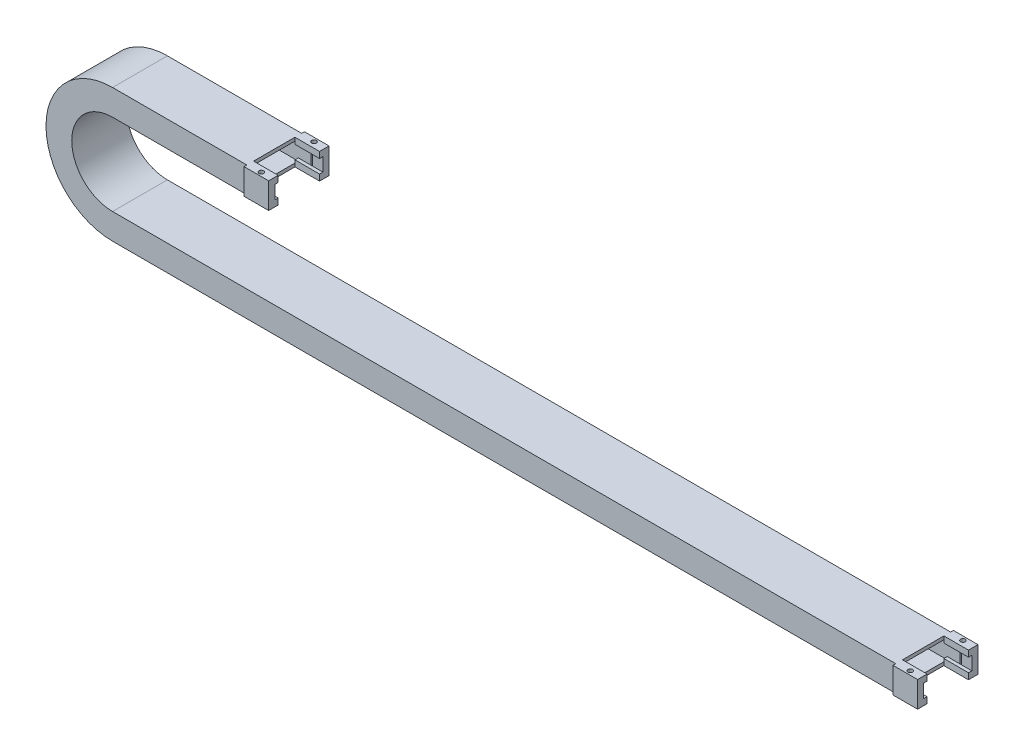
SolidWorks part; units mm, degrees
ref_plane "前视基准面" through (0, 0, 0) normal (0, 0, 1) x (1, 0, 0)
ref_plane "上视基准面" through (0, 0, 0) normal (0, 1, 0) x (1, 0, 0)
ref_plane "右视基准面" through (0, 0, 0) normal (1, 0, 0) x (0, 0, -1)
sketch "草图1" plane through (0, 0, 0) normal (0, 0, 1) x (1, 0, 0)
  line L0 (0, 0) -> (-700, 0)
  line L1 (-700, 96) -> (-580, 96)
  arc A0 (-700, 96) -> (-700, 0) centre (-700, 48) ccw
  dimension "D2" = 48
  dimension "D1" = 700
  dimension "D3" = 120
sketch "草图2" plane through (0, 0, 0) normal (1, 0, 0) x (0, 0, -1)
  line L1 (24.5, 11.5) -> (-24.5, 11.5)
  line L2 (24.5, 11.5) -> (24.5, -11.5)
  line L3 (24.5, -11.5) -> (-24.5, -11.5)
  line L4 (-24.5, 11.5) -> (-24.5, -11.5)
  line L5 (24.5, 11.5) -> (-24.5, -11.5) construction
  line L6 (24.5, -11.5) -> (-24.5, 11.5) construction
  point P0 (0, 0)
  dimension "D1" = 23
  dimension "D2" = 49
sweep "扫描1" add profiles "草图2" path "草图1"
shell "抽壳1" thickness 3
sketch "草图3" plane through (0, 11.5, 0) normal (0, 1, 0) x (1, 0, 0)
  line L0 (-7, 7.5) -> (-7, -7.5) construction
  line L1 (0, 0) -> (-7, 0) construction
  line L2 (0, 24.5) -> (0, -24.5) construction
  circle A0 centre (-7, 7.5) radius 2.5
  circle A1 centre (-7, -7.5) radius 2.5
  dimension "D2" = 7
  dimension "D1" = 5
  dimension "D3" = 15
extrude "切除-拉伸1" [suppressed] cut sketch "草图3" against normal through all
sketch "草图4" plane through (0, 107.5, 0) normal (0, 1, 0) x (1, 0, 0)
  line L0 (-587, 7.5) -> (-587, -7.5) construction
  line L1 (-587, 0) -> (-580, 0) construction
  line L2 (-580, -24.5) -> (-580, 24.5) construction
  circle A0 centre (-587, 7.5) radius 2.5
  circle A1 centre (-587, -7.5) radius 2.5
  dimension "D1" = 15
  dimension "D2" = 5
  dimension "D3" = 7
extrude "切除-拉伸2" [suppressed] cut sketch "草图4" against normal up to surface (24 mm away)
sketch "草图5" plane through (0, 11.5, 0) normal (0, 1, 0) x (1, 0, 0)
  line L0 (0, 24.5) -> (0, -24.5) construction
  line L1 (-40, 21) -> (25.9694, 21)
  line L2 (-40, 21) -> (-40, -21)
  line L3 (-40, -21) -> (25.9694, -21)
  line L4 (25.9694, 21) -> (25.9694, -21)
  line L5 (-40, 21) -> (25.9694, -21) construction
  line L6 (-40, -21) -> (25.9694, 21) construction
  point P0 (-7.0153, 0)
  dimension "D1" = 42
  dimension "D2" = 40
extrude "切除-拉伸3" [suppressed] cut sketch "草图5" against normal blind 5
sketch "草图6" plane through (0, 0, 24.5) normal (0, 0, 1) x (1, 0, 0)
  line L0 (-20, 11.5) -> (0, 1.5)
  line L1 (-700, 11.5) -> (0, 11.5) construction
  line L2 (0, 11.5) -> (0, -11.5) construction
  line L3 (0, 1.5) -> (0, 11.5)
  line L4 (0, 11.5) -> (-20, 11.5)
  dimension "D1" = 20
  dimension "D2" = 10
extrude "切除-拉伸4" [suppressed] cut sketch "草图6" against normal through all
fillet "圆角1" [suppressed] radius 5
sketch "草图7" plane through (0, -8.5, 0) normal (0, 1, 0) x (1, 0, 0)
  line L0 (0, -21.5) -> (0, 21.5) construction
  line L1 (-39, 18.5) -> (-25, 18.5)
  line L2 (-39, 18.5) -> (-39, -18.5)
  line L3 (-39, -18.5) -> (-25, -18.5)
  line L4 (-25, 18.5) -> (-25, -18.5)
  line L5 (-39, 18.5) -> (-25, -18.5) construction
  line L6 (-39, -18.5) -> (-25, 18.5) construction
  point P0 (-32, 0)
  dimension "D1" = 14
  dimension "D2" = 37
  dimension "D3" = 25
extrude "切除-拉伸5" [suppressed] cut sketch "草图7" against normal blind 5
sketch "草图8" plane through (0, 104.5, 0) normal (0, -1, 0) x (1, 0, 0)
  line L0 (-580, -24.5) -> (-580, 24.5) construction
  line L1 (-620, 21) -> (-279.3779, 21)
  line L2 (-620, 21) -> (-620, -21)
  line L3 (-620, -21) -> (-279.3779, -21)
  line L4 (-279.3779, 21) -> (-279.3779, -21)
  line L5 (-620, 21) -> (-279.3779, -21) construction
  line L6 (-620, -21) -> (-279.3779, 21) construction
  point P0 (-449.689, 0)
  dimension "D1" = 42
  dimension "D2" = 40
extrude "切除-拉伸6" [suppressed] cut sketch "草图8" against normal blind 5
sketch "草图9" plane through (0, 0, 24.5) normal (0, 0, 1) x (1, 0, 0)
  line L0 (-580, 97.5) -> (-580, 107.5)
  line L1 (-580, 84.5) -> (-580, 107.5) construction
  line L3 (-580, 107.5) -> (-600, 107.5)
  line L4 (-700, 107.5) -> (-580, 107.5) construction
  line L5 (-600, 107.5) -> (-580, 97.5)
  dimension "D1" = 10
  dimension "D2" = 20
extrude "切除-拉伸7" [suppressed] cut sketch "草图9" against normal through all
fillet "圆角2" [suppressed] radius 5
sketch "草图10" plane through (0, 87.5, 0) normal (0, 1, 0) x (1, 0, 0)
  line L0 (-580, -24.5) -> (-580, 24.5) construction
  line L1 (-605, -18.5) -> (-619, -18.5)
  line L2 (-605, -18.5) -> (-605, 18.5)
  line L3 (-605, 18.5) -> (-619, 18.5)
  line L4 (-619, -18.5) -> (-619, 18.5)
  line L5 (-605, -18.5) -> (-619, 18.5) construction
  line L6 (-605, 18.5) -> (-619, -18.5) construction
  point P0 (-612, 0)
  dimension "D1" = 37
  dimension "D2" = 14
  dimension "D3" = 25
extrude "切除-拉伸8" [suppressed] cut sketch "草图10" against normal blind 5
sketch "草图11" plane through (0, 0, 0) normal (1, 0, 0) x (0, 0, -1)
  line L0 (24.5, 11.5) -> (-24.5, 11.5) construction
  line L1 (-27, 11.5) -> (27, 11.5)
  line L2 (-27, 11.5) -> (-27, -11.5)
  line L3 (-27, -11.5) -> (27, -11.5)
  line L4 (27, 11.5) -> (27, -11.5)
  line L5 (-27, 11.5) -> (27, -11.5) construction
  line L6 (-27, -11.5) -> (27, 11.5) construction
  line L7 (-21.5, 6) -> (21.5, 6)
  line L8 (21.5, 6) -> (21.5, -6)
  line L9 (-21.5, -6) -> (21.5, -6)
  line L10 (-21.5, 6) -> (-21.5, -6)
  point P0 (0, 0)
  dimension "D1" = 54
  dimension "D2" = 5.5
extrude "凸台-拉伸1" add sketch "草图11" along normal blind 22
sketch "草图12" plane through (0, 11.5, 0) normal (0, 1, 0) x (1, 0, 0)
  line L0 (22, 27) -> (22, -27) construction
  line L1 (0, 18.5) -> (23.0119, 18.5)
  line L2 (0, 18.5) -> (0, -18.5)
  line L3 (0, -18.5) -> (23.0119, -18.5)
  line L4 (23.0119, 18.5) -> (23.0119, -18.5)
  line L5 (0, 18.5) -> (23.0119, -18.5) construction
  line L6 (0, -18.5) -> (23.0119, 18.5) construction
  point P0 (11.506, 0)
  dimension "D1" = 37
  dimension "D2" = 22
extrude "切除-拉伸9" cut sketch "草图12" against normal through all
hole_wizard "Ø4.2 (4.2) 直径孔1" positions "草图14" profile "草图13" hole size "Ø4.2" standard "GB" end condition through all
sketch "草图14" plane through (0, 11.5, 0) normal (0, 1, 0) x (1, 0, 0)
  line L0 (12, 23.5) -> (12, -23.5) construction
  line L3 (0, 0) -> (12, 0) construction
  line L6 (22, 27) -> (22, 18.5) construction
  point P0 (12, 23.5)
  point P2 (12, -23.5)
  dimension "D1" = 47
  dimension "D2" = 10
sketch "草图13" plane through (12, 11.5, -23.5) normal (1, 0, 0) x (0, 0, 1)
  line L0 (0, 0) -> (0, 23.0001)
  line L1 (0, 23.0001) -> (2.1, 23.0001)
  line L2 (2.1, 23.0001) -> (2.1, 0)
  line L5 (2.1, 0) -> (0, 0)
  line L11 (0, -6.35) -> (0, 107.95) construction
  dimension "通孔孔直径" = 4.2
  dimension "通孔孔深度" = 23.0001
sketch "草图15" plane through (-580, 0, 0) normal (1, 0, 0) x (0, 0, -1)
  line L0 (0, 96) -> (0, 0) construction
  line L1 (-27, 107.5) -> (27, 107.5)
  line L2 (-27, 107.5) -> (-27, 84.5)
  line L3 (-27, 84.5) -> (27, 84.5)
  line L4 (27, 107.5) -> (27, 84.5)
  line L5 (-27, 107.5) -> (27, 84.5) construction
  line L6 (-27, 84.5) -> (27, 107.5) construction
  line L7 (-24.5, 107.5) -> (24.5, 107.5) construction
  line L8 (24.5, 84.5) -> (-24.5, 84.5) construction
  line L9 (-21.5, 102) -> (21.5, 102)
  line L10 (21.5, 102) -> (21.5, 90)
  line L11 (-21.5, 90) -> (21.5, 90)
  line L12 (-21.5, 102) -> (-21.5, 90)
  point P0 (0, 96)
  dimension "D1" = 54
  dimension "D2" = 5.5
extrude "凸台-拉伸2" add sketch "草图15" along normal blind 22
sketch "草图16" plane through (0, 107.5, 0) normal (0, 1, 0) x (1, 0, 0)
  line L0 (0, 0) -> (-700, 0) construction
  line L1 (-580, 18.5) -> (-534.2045, 18.5)
  line L2 (-580, 18.5) -> (-580, -18.5)
  line L3 (-580, -18.5) -> (-534.2045, -18.5)
  line L4 (-534.2045, 18.5) -> (-534.2045, -18.5)
  line L5 (-580, 18.5) -> (-534.2045, -18.5) construction
  line L6 (-580, -18.5) -> (-534.2045, 18.5) construction
  line L7 (-557.1023, 0) -> (-558, 0) construction
  line L8 (-558, 27) -> (-558, -27) construction
  point P0 (-557.1023, 0)
  dimension "D1" = 37
  dimension "D2" = 22
extrude "切除-拉伸10" cut sketch "草图16" against normal blind 49
hole_wizard "Ø4.2 (4.2) 直径孔2" positions "草图18" profile "草图17" hole size "Ø4.2" standard "GB"
sketch "草图18" plane through (0, 107.5, 0) normal (0, 1, 0) x (1, 0, 0)
  line L0 (-568, 23.5) -> (-568, -23.5) construction
  line L3 (-580, 0) -> (-568, 0) construction
  line L4 (-580, 18.5) -> (-580, -18.5) construction
  line L7 (-558, 27) -> (-558, 18.5) construction
  point P0 (-568, 23.5)
  point P2 (-568, -23.5)
  dimension "D1" = 47
  dimension "D2" = 10
sketch "草图17" plane through (-568, 107.5, -23.5) normal (1, 0, 0) x (0, 0, 1)
  line L0 (0, 0) -> (0, 51.2618)
  line L1 (0, 51.2618) -> (2.1, 50)
  line L2 (2.1, 50) -> (2.1, 0)
  line L5 (2.1, 0) -> (0, 0)
  line L10 (0, 51.2618) -> (-2.1, 50) construction
  line L11 (0, -6.35) -> (0, 107.95) construction
  dimension "孔直径" = 4.2
  dimension "孔深度" = 50
  dimension "导头角度" = 118
